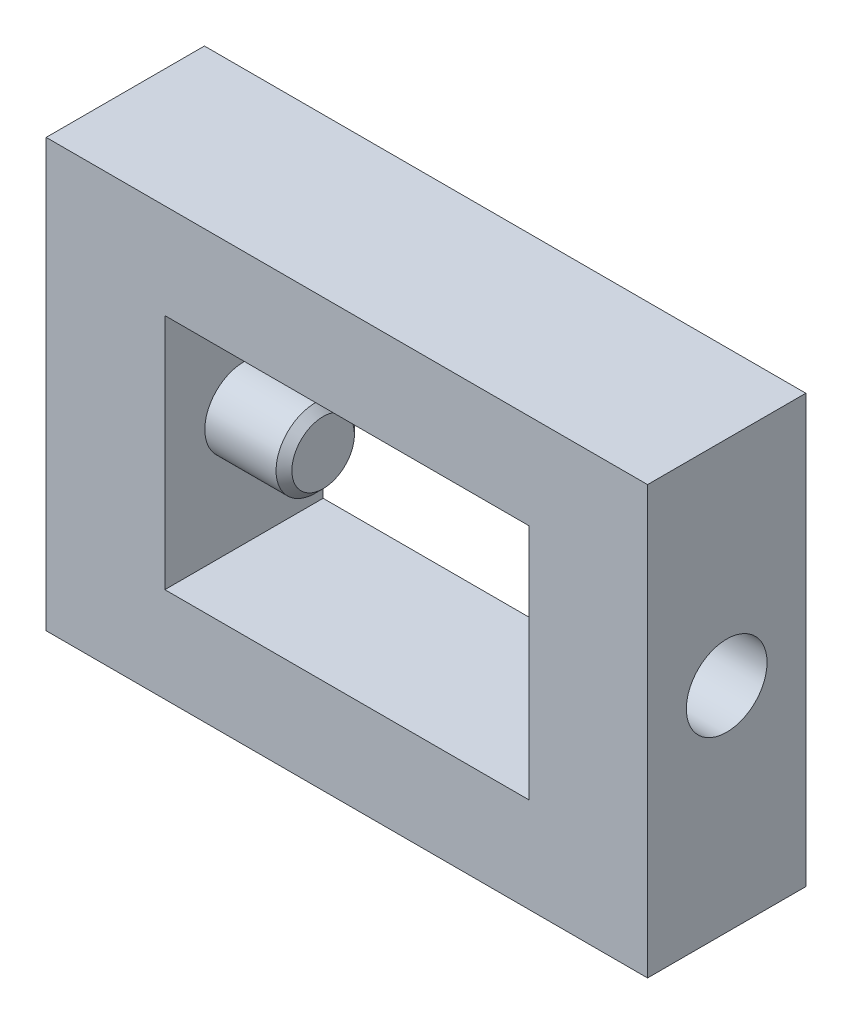
SolidWorks part; units mm, degrees
material "A3"
ref_plane "前视基准面" through (0, 0, 0) normal (0, 0, 1) x (1, 0, 0)
ref_plane "上视基准面" through (0, 0, 0) normal (0, 1, 0) x (1, 0, 0)
ref_plane "右视基准面" through (0, 0, 0) normal (1, 0, 0) x (0, 0, -1)
sketch "草图1" plane through (0, 0, 0) normal (0, 0, 1) x (1, 0, 0)
  line L1 (-38, -27) -> (38, -27)
  line L2 (-38, -27) -> (-38, 27)
  line L3 (-38, 27) -> (38, 27)
  line L4 (38, -27) -> (38, 27)
  line L5 (-38, -27) -> (38, 27) construction
  line L6 (-38, 27) -> (38, -27) construction
  line L7 (23, 15) -> (-23, 15)
  line L8 (23, 15) -> (23, -15)
  line L9 (23, -15) -> (-23, -15)
  line L10 (-23, 15) -> (-23, -15)
  line L11 (23, 15) -> (-23, -15) construction
  line L12 (23, -15) -> (-23, 15) construction
  point P0 (0, 0)
  point P5 (0, 0)
  dimension "D1" = 54
  dimension "D2" = 76
  dimension "D3" = 30
  dimension "D4" = 46
extrude "凸台-拉伸1" add sketch "草图1" along normal mid plane 20
sketch "草图2" plane through (-38, 0, 0) normal (-1, 0, 0) x (0, 0, 1)
  circle A0 centre (0, 0) radius 4.95
  dimension "D1" = 9.9
extrude "切除-拉伸1" cut sketch "草图2" against normal blind 20
hole_wizard "M12 螺纹孔1" positions "草图3" profile "草图4" tap size "M12" standard "GB"
sketch "草图3" plane through (38, 0, 0) normal (1, 0, 0) x (0, 0, -1)
  point P0 (0, 0)
sketch "草图4" plane through (38, 0, 0) normal (0, 1, 0) x (0, 0, -1)
  line L0 (0, 0) -> (0, 35.8144)
  line L1 (0, 35.8144) -> (5.1, 32.75)
  line L2 (5.1, 32.75) -> (5.1, 0)
  line L5 (5.1, 0) -> (0, 0)
  line L10 (0, 35.8144) -> (-5.1, 32.75) construction
  line L11 (0, -6.35) -> (0, 107.95) construction
  dimension "螺纹孔钻头直径" = 10.2
  dimension "螺纹孔钻头深度" = 32.75
  dimension "导头角度" = 118
cosmetic thread "孔螺蚊线1" parameters "D1"=24, "D2"=12
sketch "草图5" plane through (-38, 0, 0) normal (-1, 0, 0) x (0, 0, 1)
  circle A0 centre (0, 0) radius 4.95 construction
  circle A1 centre (0, 0) radius 4.95
extrude "凸台-拉伸2" add sketch "草图5" against normal blind 25 separate body
chamfer "倒角1" distance 1 angle 45 2 edges at (-38, -4.95, 0) (-13, -4.95, 0)
